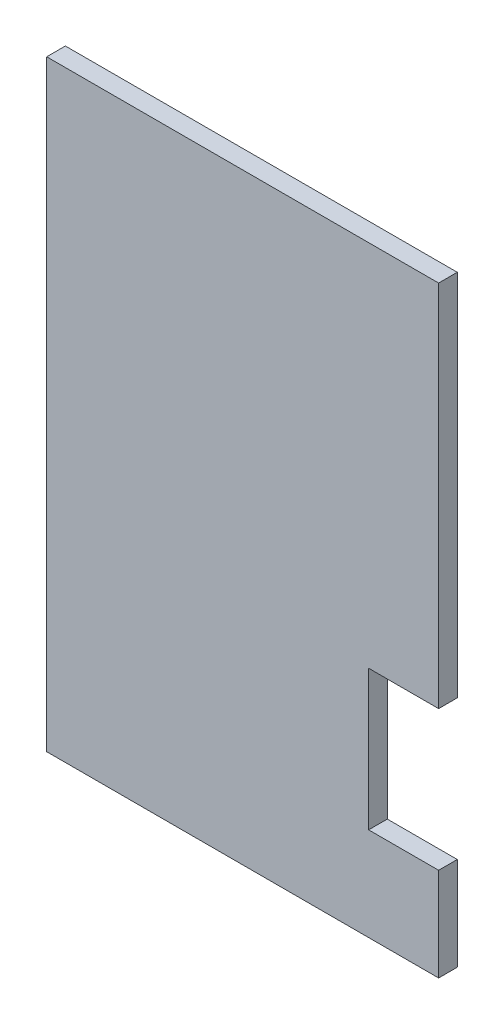
from build123d import *

# Parameters (mm, degrees)
BOSS_EXTRUDE1_DEPTH = 40


with BuildPart() as part:
    # Sketch1 → Boss-Extrude1 (new body)
    with BuildSketch(Plane.XY):
        Polygon((0, 0), (840, 0), (840, 200), (690, 200), (690, 500), (840, 500), (840, 1290), (0, 1290), align=None)
    extrude(amount=BOSS_EXTRUDE1_DEPTH)


solid = part.part
